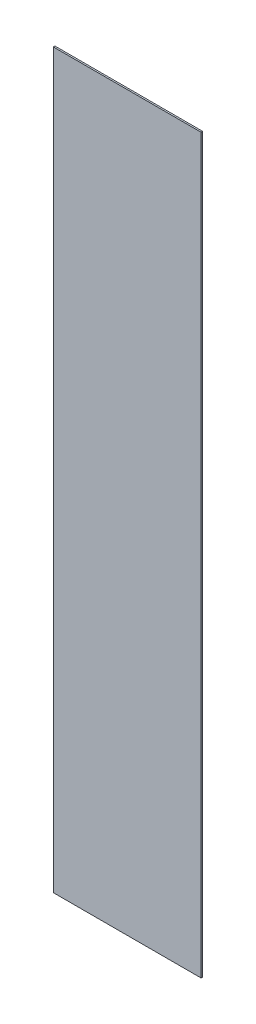
SolidWorks part; units mm, degrees
material "PMMA(有机玻璃)"
ref_plane "前视" through (0, 0, 0) normal (0, 0, 1) x (1, 0, 0)
ref_plane "上视" through (0, 0, 0) normal (0, 1, 0) x (1, 0, 0)
ref_plane "右视" through (0, 0, 0) normal (1, 0, 0) x (0, 0, -1)
sketch "草图1" plane through (0, 0, 0) normal (0, 0, 1) x (1, 0, 0)
  line L1 (-233, 1155) -> (233, 1155)
  line L2 (-233, 1155) -> (-233, -1155)
  line L3 (-233, -1155) -> (233, -1155)
  line L4 (233, 1155) -> (233, -1155)
  line L5 (-233, 1155) -> (233, -1155) construction
  line L6 (-233, -1155) -> (233, 1155) construction
  point P0 (0, 0)
  dimension "D1" = 2310
  dimension "D2" = 466
extrude "凸台-拉伸1" add sketch "草图1" along normal blind 5
hole_wizard "M5 间隙孔1" positions "草图3" profile "草图2" hole size "M5" standard "GB"
sketch "草图3" plane through (0, 0, 5) normal (0, 0, 1) x (1, 0, 0)
  line L0 (-427.5, 273) -> (-427.5, -273) construction
  line L1 (-427.5, -273) -> (427.5, -273) construction
  line L2 (0, 273) -> (0, -273) construction
  line L3 (427.5, 273) -> (-427.5, 273) construction
  line L5 (-427.5, 0) -> (427.5, 0) construction
  line L6 (427.5, -273) -> (427.5, 273) construction
  point P0 (-375, -261)
  point P46 (415.5, 250)
  point P48 (-415.5, 250)
  point P58 (-125, -261)
  point P59 (125, -261)
  point P61 (-125, 261)
  point P62 (125, 261)
  point P64 (-375, 261)
  point P88 (375, -261)
  point P89 (375, 261)
  point P108 (415.5, 0)
  point P109 (-415.5, 0)
  point P110 (415.5, -250)
  point P111 (-415.5, -250)
  dimension "D1" = 12
  dimension "D2" = 12
  dimension "D5" = 3
  dimension "D3" = 12
  dimension "D6" = 4
  dimension "D4" = 2
sketch "草图2" plane through (-375, -261, 5) normal (1, 0, 0) x (0, -1, 0)
  line L0 (0, 0) -> (0, 5)
  line L1 (0, 5) -> (2.75, 5)
  line L2 (2.75, 5) -> (2.75, 0)
  line L5 (2.75, 0) -> (0, 0)
  line L11 (0, -6.35) -> (0, 107.95) construction
  dimension "通孔孔直径" = 5.5
  dimension "通孔孔深度" = 5
